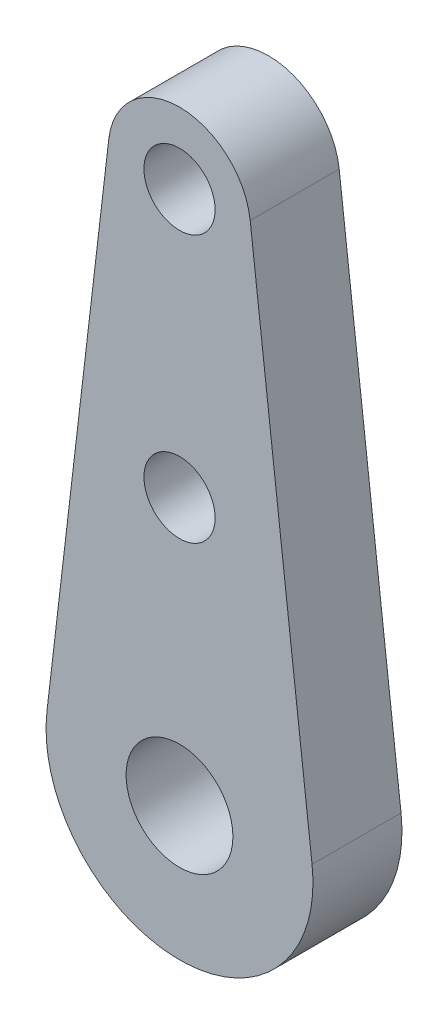
from build123d import *

# Parameters (mm, degrees)
SKETCH1_R           = 2
SKETCH1_R_2         = 3
BOSS_EXTRUDE1_DEPTH = 5
SKETCH2_R           = 2
CUT_EXTRUDE1_DEPTH  = 36.174564674


with BuildPart() as part:
    # Sketch1 → Boss-Extrude1 (new body)
    with BuildSketch(Plane.XY):
        with BuildLine():
            Line((-3.972684511, 30.466666667), (-7.448783458, 0.875))
            ThreePointArc((-7.448783458, 0.875), (0, -7.5), (7.448783458, 0.875))
            Line((7.448783458, 0.875), (3.972684511, 30.466666667))
            ThreePointArc((3.972684511, 30.466666667), (0, 34), (-3.972684511, 30.466666667))
        make_face()
        with Locations((0, 30)):
            Circle(SKETCH1_R, mode=Mode.SUBTRACT)
        Circle(SKETCH1_R_2, mode=Mode.SUBTRACT)
    extrude(amount=BOSS_EXTRUDE1_DEPTH)

    # Sketch2 → Cut-Extrude1 (cut, through all)
    with BuildSketch(Plane.XY.offset(5)):
        with Locations((0, 15)):
            Circle(SKETCH2_R)
    extrude(amount=-CUT_EXTRUDE1_DEPTH, mode=Mode.SUBTRACT)


solid = part.part
